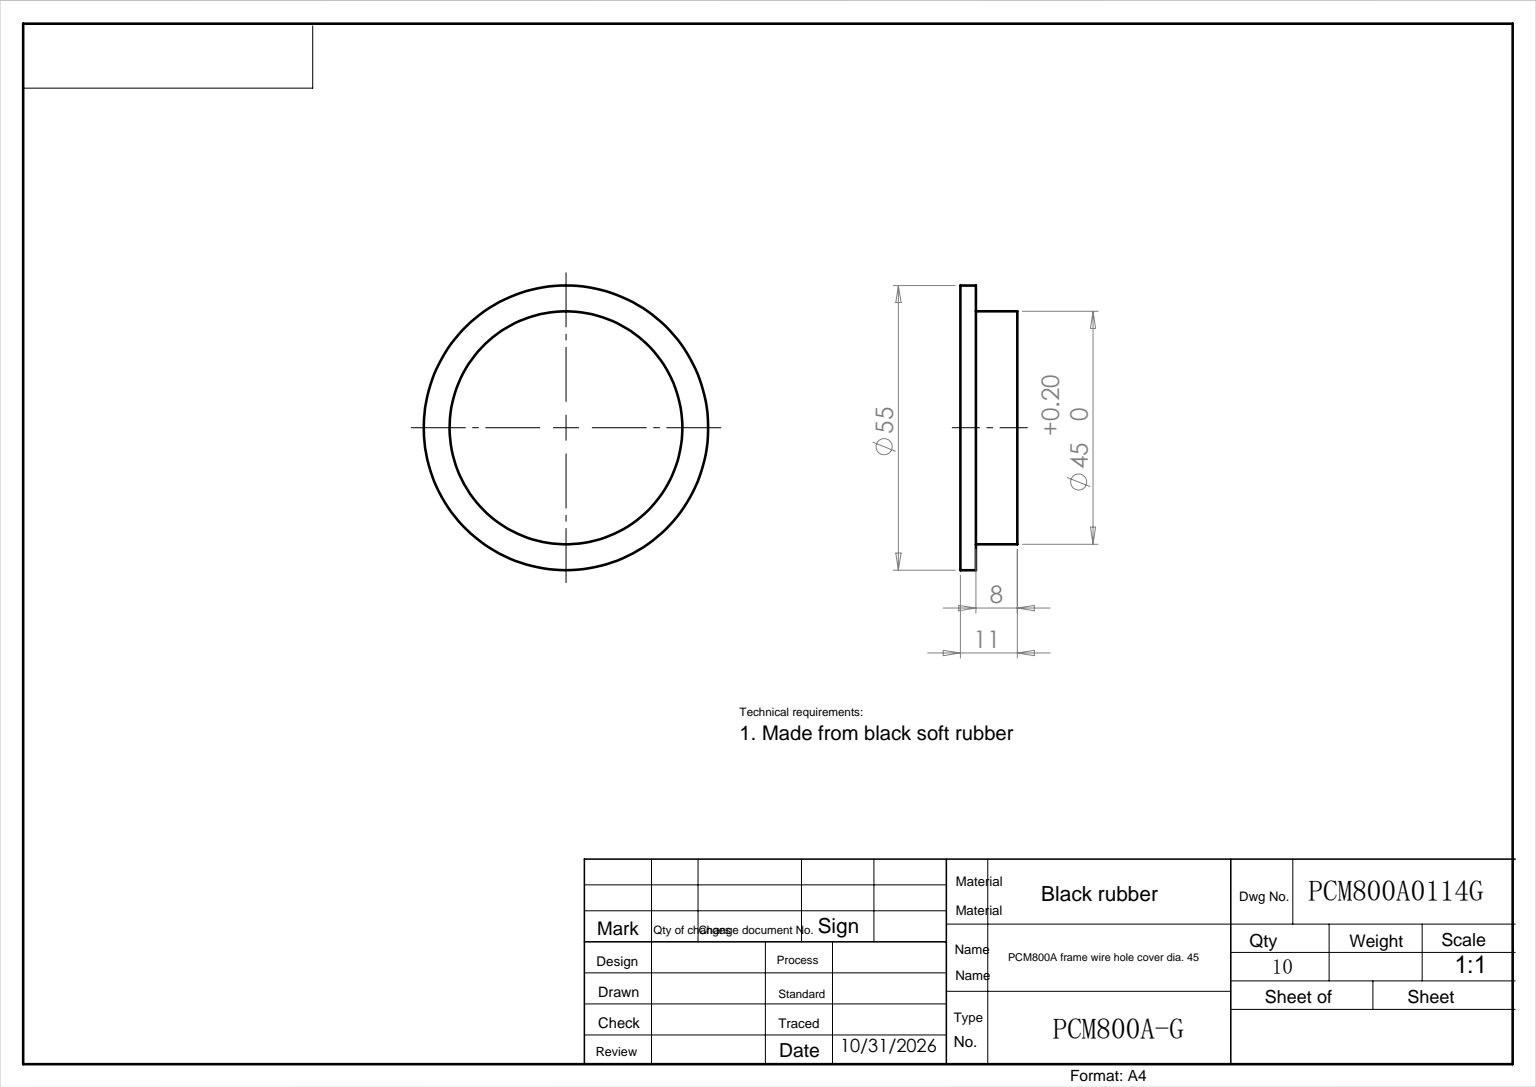
SolidWorks part; units mm, degrees
ref_plane "前视基准面" through (0, 0, 0) normal (0, 0, 1) x (1, 0, 0)
ref_plane "上视基准面" through (0, 0, 0) normal (0, 1, 0) x (1, 0, 0)
ref_plane "右视基准面" through (0, 0, 0) normal (1, 0, 0) x (0, 0, -1)
sketch "草图1" plane through (0, 0, 0) normal (0, 0, 1) x (1, 0, 0)
  line L0 (0, 0) -> (0, 78.3105) construction
  line L1 (0, 0) -> (71.1603, 0) construction
  line L2 (0, 0) -> (-27.5, 0)
  line L3 (-27.5, 0) -> (-27.5, 3)
  line L4 (-27.5, 3) -> (-22.5, 3)
  line L5 (-22.5, 3) -> (-22.5, 11)
  line L6 (-22.5, 11) -> (0, 11)
  line L7 (0, 11) -> (0, 0)
  dimension "D1" = 22.5
  dimension "D2" = 27.5
  dimension "D3" = 3
  dimension "D4" = 8
revolve "旋转1" add sketch "草图1" angle 180 about L0 other way angle 180
